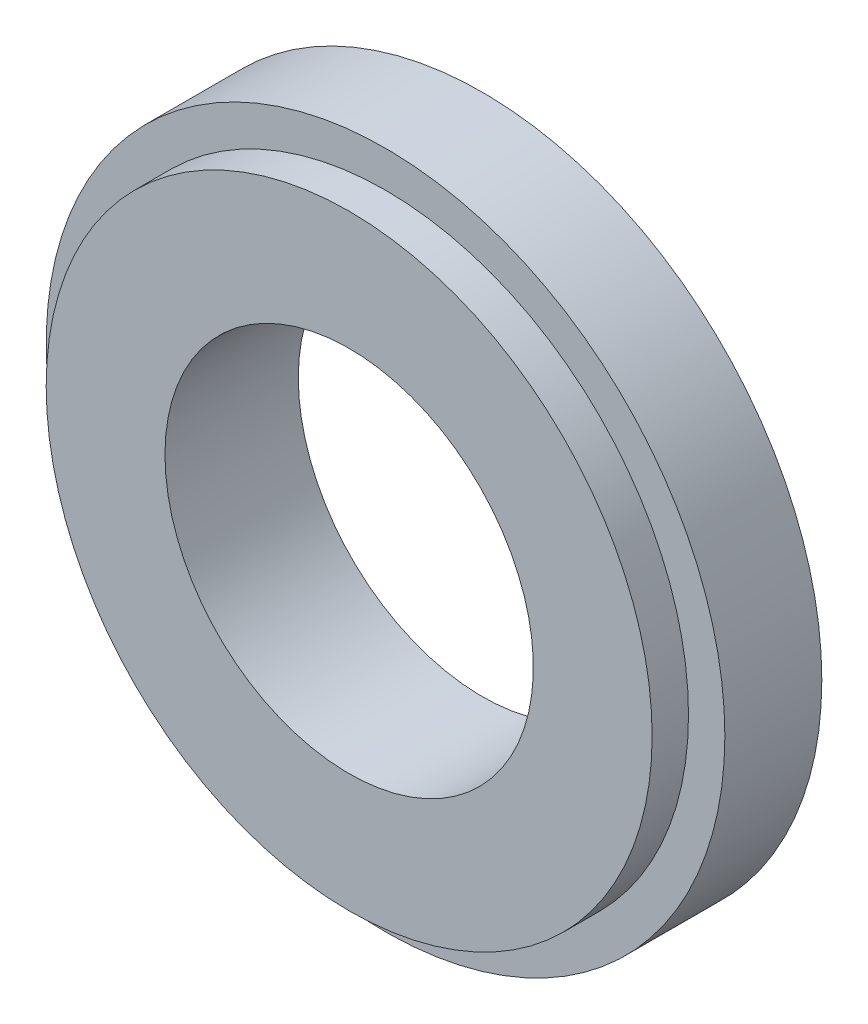
SolidWorks part; units mm, degrees
ref_plane "Front Plane" through (0, 0, 0) normal (0, 0, 1) x (1, 0, 0)
ref_plane "Top Plane" through (0, 0, 0) normal (0, 1, 0) x (1, 0, 0)
ref_plane "Right Plane" through (0, 0, 0) normal (1, 0, 0) x (0, 0, -1)
sketch "Sketch1" plane through (0, 0, 0) normal (0, 0, 1) x (1, 0, 0)
  circle A0 centre (0, 0) radius 28
extrude "Boss-Extrude1" add sketch "Sketch1" along normal blind 8
sketch "Sketch2" plane through (0, 0, 8) normal (0, 0, 1) x (1, 0, 0)
  circle A0 centre (0, 0) radius 25
extrude "Boss-Extrude2" add sketch "Sketch2" along normal blind 3
sketch "Sketch4" plane through (0, 0, 0) normal (0, 0, -1) x (-1, 0, 0)
  circle A0 centre (0, 0) radius 15.1985
extrude "Cut-Extrude1" cut sketch "Sketch4" against normal through all
